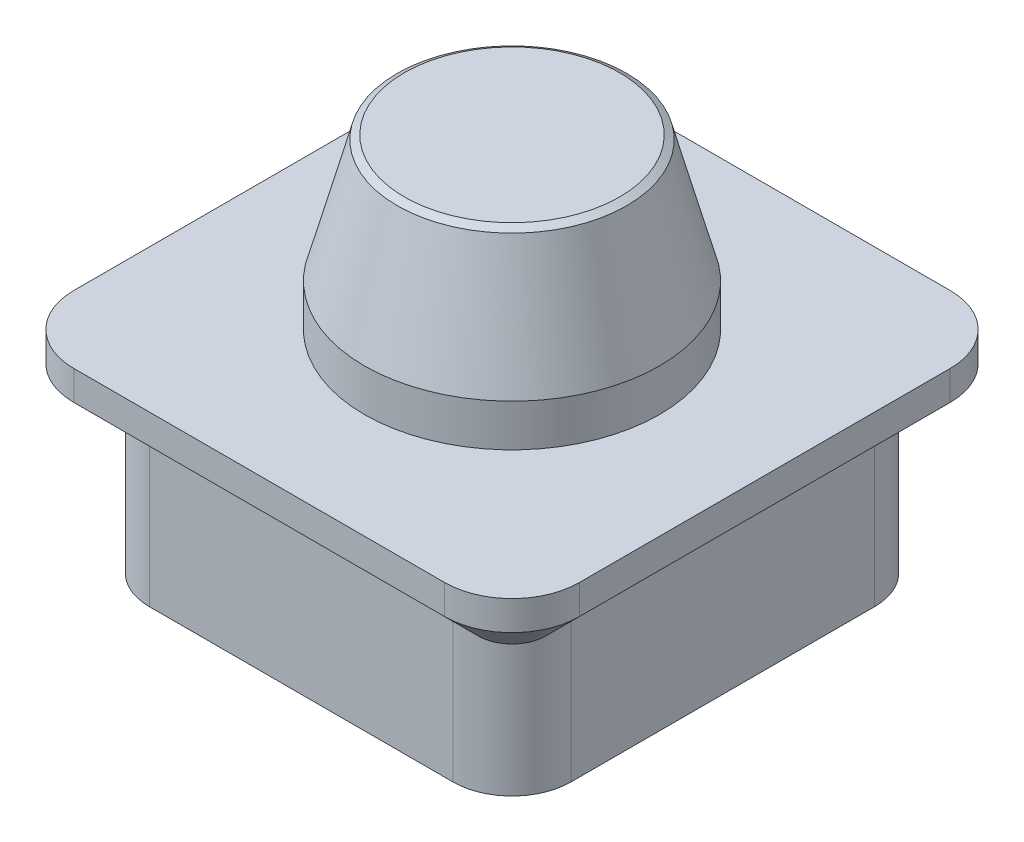
SolidWorks part; units mm, degrees
material "Q235B"
ref_plane "Front Plane" through (0, 0, 0) normal (0, 0, 1) x (1, 0, 0)
ref_plane "Top Plane" through (0, 0, 0) normal (0, 1, 0) x (1, 0, 0)
ref_plane "Right Plane" through (0, 0, 0) normal (1, 0, 0) x (0, 0, -1)
sketch "feature 17 (ProfileFeature) (+16 more in 12 files) Sketch1" plane through (0, 0, 0) normal (0, 0, 1) x (1, 0, 0)
  line L0 (0, 0) -> (35, 0)
  line L1 (35, 0) -> (35, 10)
  line L2 (35, 10) -> (26.9615, 40)
  line L3 (26.9615, 40) -> (0, 40)
  line L4 (0, 40) -> (0, -18.6749) construction
  line L5 (0, 0) -> (0, 40)
  dimension "D1" = 70
  dimension "D2" = 15
  dimension "D3" = 10
  dimension "D4" = 40
revolve "Revolve1" add sketch "feature 17 (ProfileFeature) (+16 more in 12 files) Sketch1" angle 360 about L4
chamfer "Chamfer1" distance 1 angle 45 1 edges at (-26.9615, 40, 0)
sketch "0:feat:20/0 feature 20/0 (ProfileFeature) (+11 more in 7 files) Sketch2" plane through (0, 0, 0) normal (0, -1, 0) x (1, 0, 0)
  line L1 (44, -60) -> (-44, -60)
  line L2 (60, -44) -> (60, 44)
  line L3 (44, 60) -> (-44, 60)
  line L4 (-60, -44) -> (-60, 44)
  line L5 (60, -60) -> (-60, 60) construction
  line L6 (60, 60) -> (-60, -60) construction
  arc A0 (-44, -60) -> (-60, -44) centre (-44, -44) cw
  arc A1 (60, 44) -> (44, 60) centre (44, 44) ccw
  arc A2 (44, -60) -> (60, -44) centre (44, -44) ccw
  arc A3 (-44, 60) -> (-60, 44) centre (-44, 44) ccw
  point P0 (0, 0)
  dimension "D2" = 16
  dimension "D1" = 120
extrude "Boss-Extrude1" add sketch "0:feat:20/0 feature 20/0 (ProfileFeature) (+11 more in 7 files) Sketch2" along normal blind 15
sketch "0:feat:20/1 feature 20/1 (ProfileFeature) (+2 more in 2 files) Sketch3" plane through (0, -15, 0) normal (0, -1, 0) x (1, 0, 0)
  line L1 (36, -50) -> (-36, -50)
  line L2 (50, -36) -> (50, 36)
  line L3 (36, 50) -> (-36, 50)
  line L4 (-50, -36) -> (-50, 36)
  line L5 (50, -50) -> (-50, 50) construction
  line L6 (50, 50) -> (-50, -50) construction
  arc A0 (-36, -50) -> (-50, -36) centre (-36, -36) cw
  arc A1 (50, 36) -> (36, 50) centre (36, 36) ccw
  arc A2 (36, -50) -> (50, -36) centre (36, -36) ccw
  arc A3 (-36, 50) -> (-50, 36) centre (-36, 36) ccw
  point P0 (0, 0)
  dimension "D2" = 14
  dimension "D1" = 100
extrude "Boss-Extrude2" add sketch "0:feat:20/1 feature 20/1 (ProfileFeature) (+2 more in 2 files) Sketch3" along normal blind 35
chamfer "Chamfer2" distance 8 angle 45 8 edges at (-55.3137, -15, -55.3137) (0, -15, -60) (-60, -15, 0) (55.3137, -15, -55.3137) (-55.3137, -15, 55.3137) (60, -15, 0) (0, -15, 60) (55.3137, -15, 55.3137)
